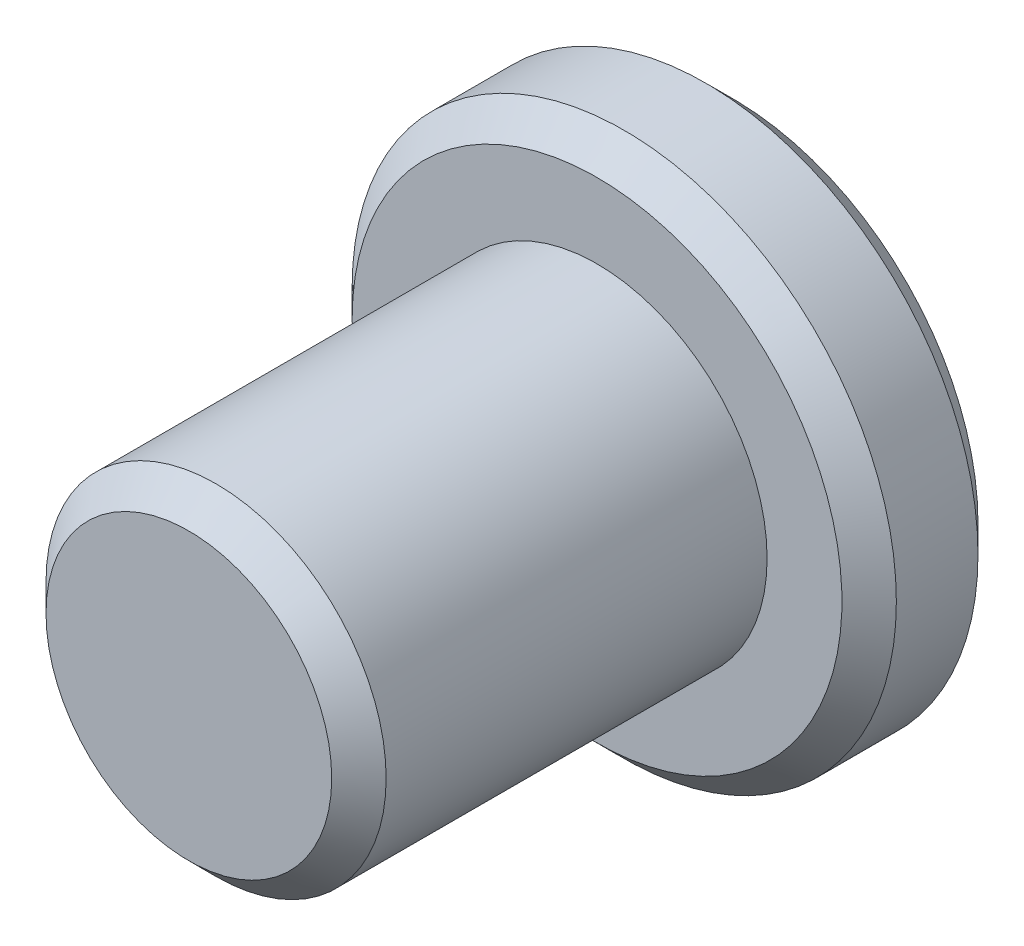
from build123d import *

# Parameters (mm, degrees)
CHAMFER1_SIZE = 1


with BuildPart() as part:
    # Sketch1 → Revolve1 (revolve)
    with BuildSketch(Plane(origin=(0, 0, 0), x_dir=(0, 0, -1), z_dir=(1, 0, 0)), mode=Mode.PRIVATE) as revolve1_sk:
        Polygon((20, 0), (20, 10), (15, 10), (15, 6.25), (0, 6.25), (0, 0), align=None)
    revolve(revolve1_sk.sketch.rotate(Axis((0, 0, 0), (0, 0, -1)), 90), axis=Axis((0, 0, 0), (0, 0, -1)))

    # Chamfer1
    chamfer1_edges = [part.edges().sort_by_distance(p)[0] for p in [
        (-6.25, 0, 0),
        (-10, 0, -15),
        (-10, 0, -20),
    ]]
    chamfer(chamfer1_edges, length=CHAMFER1_SIZE)


solid = part.part
